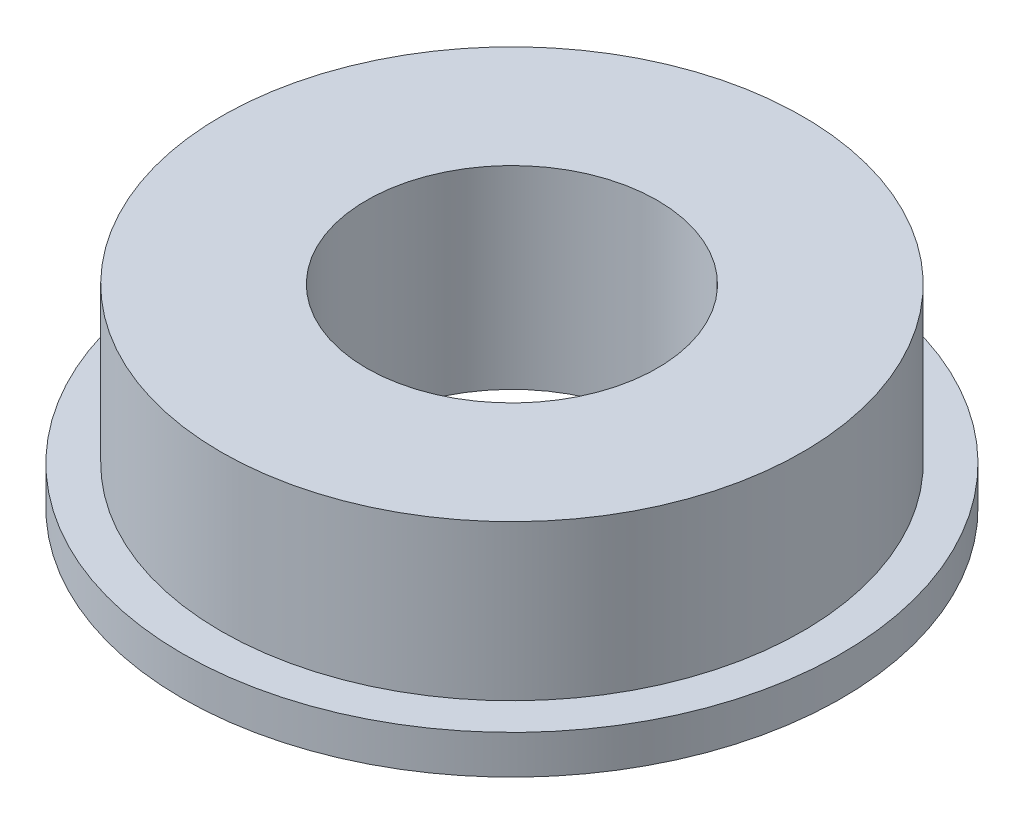
SolidWorks part; units mm, degrees
material "镀铬不锈钢"
ref_plane "前视基准面" through (0, 0, 0) normal (0, 0, 1) x (1, 0, 0)
ref_plane "上视基准面" through (0, 0, 0) normal (0, 1, 0) x (1, 0, 0)
ref_plane "右视基准面" through (0, 0, 0) normal (1, 0, 0) x (0, 0, -1)
sketch "草图1" plane through (0, 0, 0) normal (0, 1, 0) x (1, 0, 0)
  circle A0 centre (0, 0) radius 6.8
  circle A1 centre (0, 0) radius 3
  dimension "D1" = 6
  dimension "D2" = 13.6
extrude "凸台-拉伸1" add sketch "草图1" along normal blind 0.8
sketch "草图2" plane through (0, 0.8, 0) normal (0, 1, 0) x (1, 0, 0)
  circle A0 centre (0, 0) radius 3 construction
  circle A1 centre (0, 0) radius 3
  circle A2 centre (0, 0) radius 6
  dimension "D1" = 12
extrude "凸台-拉伸2" add sketch "草图2" along normal blind 3.2
